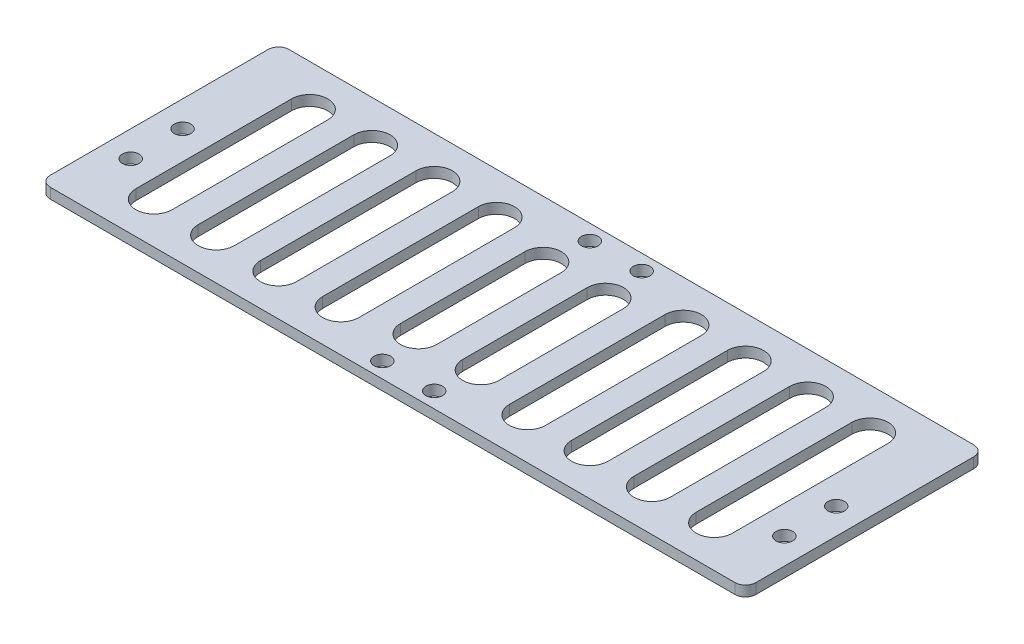
SolidWorks part; units mm, degrees
material "Thornel Mat VMA"
ref_plane "Front Plane" through (0, 0, 0) normal (0, 0, 1) x (1, 0, 0)
ref_plane "Top Plane" through (0, 0, 0) normal (0, 1, 0) x (1, 0, 0)
ref_plane "Right Plane" through (0, 0, 0) normal (1, 0, 0) x (0, 0, -1)
sketch "Sketch1" plane through (0, 0, 0) normal (0, 1, 0) x (1, 0, 0)
  line L0 (0, 23) -> (0, -23) construction
  line L1 (68, -23) -> (-68, -23)
  line L2 (68, -23) -> (68, 23)
  line L3 (68, 23) -> (-68, 23)
  line L4 (-68, -23) -> (-68, 23)
  line L5 (68, -23) -> (-68, 23) construction
  line L6 (68, 23) -> (-68, -23) construction
  line L7 (-63, -0.5) -> (-63, -10.5) construction
  line L8 (-5, -20) -> (5, -20) construction
  line L10 (63, -0.5) -> (63, -10.5) construction
  line L11 (-68, 0) -> (68, 0) construction
  line L13 (-5, 20) -> (5, 20) construction
  circle A0 centre (-63, -0.5) radius 1.6
  circle A1 centre (-63, -10.5) radius 1.6
  circle A2 centre (-5, -20) radius 1.6
  circle A3 centre (5, -20) radius 1.6
  circle A6 centre (63, -10.5) radius 1.6
  circle A7 centre (63, -0.5) radius 1.6
  circle A10 centre (5, 20) radius 1.6
  circle A11 centre (-5, 20) radius 1.6
  point P0 (0, 0)
  dimension "D2" = 12.5
  dimension "D4" = 3.2
  dimension "D1" = 136
  dimension "D3" = 10
  dimension "D5" = 5
  dimension "D6" = 3
  dimension "D7" = 46
extrude "Boss-Extrude1" add sketch "Sketch1" along normal blind 2
sketch "Sketch2" plane through (0, 2, 0) normal (0, 1, 0) x (1, 0, 0)
  line L0 (0, 23) -> (0, -23) construction
  line L1 (68, 23) -> (-68, 23) construction
  line L2 (-68, -23) -> (68, -23) construction
  line L3 (-68, 0) -> (68, 0) construction
  line L4 (-68, 23) -> (-68, -23) construction
  line L5 (68, -23) -> (68, 23) construction
  line L6 (-54, 15) -> (-54, -15) construction
  line L7 (-50.5, 15) -> (-50.5, -15)
  line L8 (-57.5, 15) -> (-57.5, -15)
  line L9 (-42, 15) -> (-42, -15) construction
  line L10 (-38.5, 15) -> (-38.5, -15)
  line L11 (-45.5, 15) -> (-45.5, -15)
  line L12 (-30, 15) -> (-30, -15) construction
  line L13 (-26.5, 15) -> (-26.5, -15)
  line L14 (-33.5, 15) -> (-33.5, -15)
  line L15 (-18, 15) -> (-18, -15) construction
  line L16 (-14.5, 15) -> (-14.5, -15)
  line L17 (-21.5, 15) -> (-21.5, -15)
  line L18 (-6, 12) -> (-6, -12) construction
  line L19 (-2.5, 12) -> (-2.5, -12)
  line L20 (-9.5, 12) -> (-9.5, -12)
  line L21 (6, 12) -> (6, -12) construction
  line L22 (9.5, 12) -> (9.5, -12)
  line L23 (2.5, 12) -> (2.5, -12)
  line L24 (18, 15) -> (18, -15) construction
  line L25 (21.5, 15) -> (21.5, -15)
  line L26 (14.5, 15) -> (14.5, -15)
  line L27 (30, 15) -> (30, -15) construction
  line L28 (33.5, 15) -> (33.5, -15)
  line L29 (26.5, 15) -> (26.5, -15)
  line L30 (42, 15) -> (42, -15) construction
  line L31 (45.5, 15) -> (45.5, -15)
  line L32 (38.5, 15) -> (38.5, -15)
  line L33 (54, 15) -> (54, -15) construction
  line L34 (57.5, 15) -> (57.5, -15)
  line L35 (50.5, 15) -> (50.5, -15)
  arc A0 (-50.5, 15) -> (-57.5, 15) centre (-54, 15) ccw
  arc A1 (-57.5, -15) -> (-50.5, -15) centre (-54, -15) ccw
  arc A2 (-38.5, 15) -> (-45.5, 15) centre (-42, 15) ccw
  arc A3 (-45.5, -15) -> (-38.5, -15) centre (-42, -15) ccw
  arc A4 (-26.5, 15) -> (-33.5, 15) centre (-30, 15) ccw
  arc A5 (-33.5, -15) -> (-26.5, -15) centre (-30, -15) ccw
  arc A6 (-14.5, 15) -> (-21.5, 15) centre (-18, 15) ccw
  arc A7 (-21.5, -15) -> (-14.5, -15) centre (-18, -15) ccw
  arc A8 (-2.5, 12) -> (-9.5, 12) centre (-6, 12) ccw
  arc A9 (-9.5, -12) -> (-2.5, -12) centre (-6, -12) ccw
  arc A10 (9.5, 12) -> (2.5, 12) centre (6, 12) ccw
  arc A11 (2.5, -12) -> (9.5, -12) centre (6, -12) ccw
  arc A12 (21.5, 15) -> (14.5, 15) centre (18, 15) ccw
  arc A13 (14.5, -15) -> (21.5, -15) centre (18, -15) ccw
  arc A14 (33.5, 15) -> (26.5, 15) centre (30, 15) ccw
  arc A15 (26.5, -15) -> (33.5, -15) centre (30, -15) ccw
  arc A16 (45.5, 15) -> (38.5, 15) centre (42, 15) ccw
  arc A17 (38.5, -15) -> (45.5, -15) centre (42, -15) ccw
  arc A18 (57.5, 15) -> (50.5, 15) centre (54, 15) ccw
  arc A19 (50.5, -15) -> (57.5, -15) centre (54, -15) ccw
  point P14 (-54, 0)
  point P22 (-42, 0)
  point P29 (-30, 0)
  point P36 (-18, 0)
  point P43 (-6, 0)
  point P50 (6, 0)
  point P57 (18, 0)
  point P64 (30, 0)
  point P71 (42, 0)
  point P78 (54, 0)
  dimension "D1" = 3.5
  dimension "D2" = 30
  dimension "D4" = 12
  dimension "D3" = 24
extrude "Cut-Extrude1" cut sketch "Sketch2" against normal through all
fillet "R2 Fillet 1" radius 2 4 edges at (-68, 1, 23) (68, 1, 23) (68, 1, -23) (-68, 1, -23)
